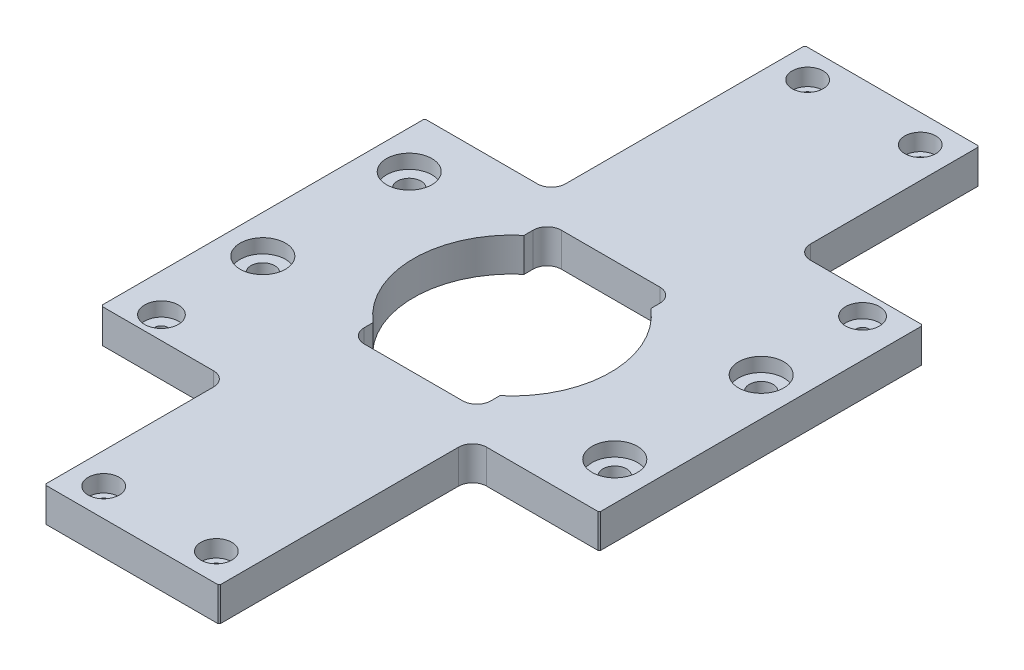
from build123d import *

# Parameters (mm, degrees)
SKETCH1_W                                            = 152
SKETCH1_H                                            = 270
BOSS_EXTRUDE1_DEPTH                                  = 6
SKETCH2_R                                            = 35
CUT_EXTRUDE1_DEPTH                                   = 156.38661461
SKETCH5_R                                            = 6
SKETCH5_R_2                                          = 8.05
CUT_EXTRUDE2_DEPTH                                   = 5
SKETCH6_W                                            = 45
SKETCH6_H                                            = 70
CUT_EXTRUDE3_DEPTH                                   = 156.38661461
SKETCH7_W                                            = 45
SKETCH7_H                                            = 90
CUT_EXTRUDE4_DEPTH                                   = 156.38661461
SKETCH8_R                                            = 7.5
CUT_EXTRUDE5_DEPTH                                   = 2
SKETCH9_W                                            = 45
SKETCH9_H                                            = 65
CUT_EXTRUDE6_DEPTH                                   = 156.38661461
FILLET1_R                                            = 5
HOLE_SIZE_PER_SOCKET_HEAD_CAP_SCREW_TYPE_D           = 6.6
HOLE_SIZE_PER_SOCKET_HEAD_CAP_SCREW_TYPE_CBORE_D     = 11
HOLE_SIZE_PER_SOCKET_HEAD_CAP_SCREW_TYPE_CBORE_DEPTH = 6
HOLE_WIZARD_2_D                                      = 4.5
HOLE_WIZARD_2_CBORE_D                                = 8
HOLE_WIZARD_2_CBORE_DEPTH                            = 4
M8_CLEARANCE_HOLE1_D                                 = 8.4
CHAMFER1_SIZE                                        = 0.5


with BuildPart() as part:
    # Sketch1 → Boss-Extrude1 (new, symmetric)
    with BuildSketch(Plane(origin=(0, 0, 0), x_dir=(1, 0, 0), z_dir=(0, 1, 0))):
        Rectangle(SKETCH1_W, SKETCH1_H)
    extrude(amount=BOSS_EXTRUDE1_DEPTH, both=True)

    # Sketch2 → Cut-Extrude1 (cut, through all)
    with BuildSketch(Plane(origin=(0, 6, 0), x_dir=(1, 0, 0), z_dir=(0, 1, 0))):
        with Locations(Location((0, 0, 0), (0, 0, 270))):
            Circle(SKETCH2_R)
    extrude(amount=-CUT_EXTRUDE1_DEPTH, mode=Mode.SUBTRACT)

    # Sketch5 → Cut-Extrude2 (cut)
    with BuildSketch(Plane(origin=(0, 6, 0), x_dir=(1, 0, 0), z_dir=(0, 1, 0))):
        with Locations(Location((62.5, 62, 0), (0, 0, 270))):
            Circle(SKETCH5_R)
        with Locations(Location((-62.5, -62, 0), (0, 0, 270))):
            Circle(SKETCH5_R)
        with Locations(Location((62.5, 26, 0), (0, 0, 270))):
            Circle(SKETCH5_R_2)
        with Locations(Location((-62.5, 26, 0), (0, 0, 90))):
            Circle(SKETCH5_R_2)
        with Locations(Location((-62.5, -26, 0), (0, 0, 270))):
            Circle(SKETCH5_R_2)
        with Locations(Location((62.5, -26, 0), (0, 0, 90))):
            Circle(SKETCH5_R_2)
    extrude(amount=-CUT_EXTRUDE2_DEPTH, mode=Mode.SUBTRACT)

    # Sketch6 → Cut-Extrude3 (cut, through all)
    with BuildSketch(Plane(origin=(0, 6, 0), x_dir=(1, 0, 0), z_dir=(0, 1, 0))):
        Rectangle(SKETCH6_W, SKETCH6_H)
    extrude(amount=-CUT_EXTRUDE3_DEPTH, mode=Mode.SUBTRACT)

    # Sketch7 → Cut-Extrude4 (cut, through all)
    with BuildSketch(Plane(origin=(0, 6, 0), x_dir=(1, 0, 0), z_dir=(0, 1, 0))):
        with Locations((-53.5, 90)):
            Rectangle(SKETCH7_W, SKETCH7_H)
        with Locations((53.5, -90)):
            Rectangle(SKETCH7_W, SKETCH7_H)
    extrude(amount=-CUT_EXTRUDE4_DEPTH, mode=Mode.SUBTRACT)

    # Sketch8 → Cut-Extrude5 (cut)
    with BuildSketch(Plane.XZ.offset(6)):
        with Locations(Location((-20, 125, 0), (0, 0, 270))):
            Circle(SKETCH8_R)
        with Locations(Location((20, 125, 0), (0, 0, 90))):
            Circle(SKETCH8_R)
        with Locations(Location((20, -125, 0), (0, 0, 270))):
            Circle(SKETCH8_R)
        with Locations(Location((-20, -125, 0), (0, 0, 90))):
            Circle(SKETCH8_R)
    extrude(amount=-CUT_EXTRUDE5_DEPTH, mode=Mode.SUBTRACT)

    # Sketch9 → Cut-Extrude6 (cut, through all)
    with BuildSketch(Plane.XZ.offset(6)):
        with Locations((-53.5, 102.5)):
            Rectangle(SKETCH9_W, SKETCH9_H)
        with Locations((53.5, -102.5)):
            Rectangle(SKETCH9_W, SKETCH9_H)
    extrude(amount=-CUT_EXTRUDE6_DEPTH, mode=Mode.SUBTRACT)

    # Fillet1
    fillet1_edges = [part.edges().sort_by_distance(p)[0] for p in [
        (-31, 0, 70),
        (31, 0, -70),
        (22.5, 0, -35),
        (22.5, 0, 35),
        (-22.5, 0, 35),
        (-22.5, 0, -35),
        (-31, 0, -45),
        (31, 0, 45),
    ]]
    fillet(fillet1_edges, radius=FILLET1_R)

    # Hole size per socket head cap screw type 2 (through all)
    with Locations(Plane(origin=(0, 6, 0), x_dir=(1, 0, 0), z_dir=(0, 1, 0))):
        with Locations((-20, 125), (20, 125), (-20, -125), (20, -125)):
            CounterBoreHole(HOLE_SIZE_PER_SOCKET_HEAD_CAP_SCREW_TYPE_D / 2, HOLE_SIZE_PER_SOCKET_HEAD_CAP_SCREW_TYPE_CBORE_D / 2, HOLE_SIZE_PER_SOCKET_HEAD_CAP_SCREW_TYPE_CBORE_DEPTH)

    # 打孔尺寸(%根据)内六角圆柱头螺钉的类型2 (through all)
    with Locations(Plane(origin=(0, -6, 0), x_dir=(-1, 0, 0), z_dir=(0, -1, 0))):
        with Locations((62.5, -62), (-62.5, 62)):
            CounterBoreHole(HOLE_WIZARD_2_D / 2, HOLE_WIZARD_2_CBORE_D / 2, HOLE_WIZARD_2_CBORE_DEPTH)

    # M8 Clearance Hole1 (through all)
    with Locations(Plane(origin=(0, -6, 0), x_dir=(-1, 0, 0), z_dir=(0, -1, 0))):
        with Locations((62.5, -26), (62.5, 26), (-62.5, -26), (-62.5, 26)):
            Hole(M8_CLEARANCE_HOLE1_D / 2)

    # Chamfer1
    chamfer1_edges = [part.edges().sort_by_distance(p)[0] for p in [
        (-76, 0, 70),
        (-31, 0, 135),
        (76, 0, -70),
        (31, 0, -135),
        (-76, 0, -45),
        (-31, 0, -135),
        (76, 0, 45),
        (31, 0, 135),
    ]]
    chamfer(chamfer1_edges, length=CHAMFER1_SIZE)


solid = part.part
